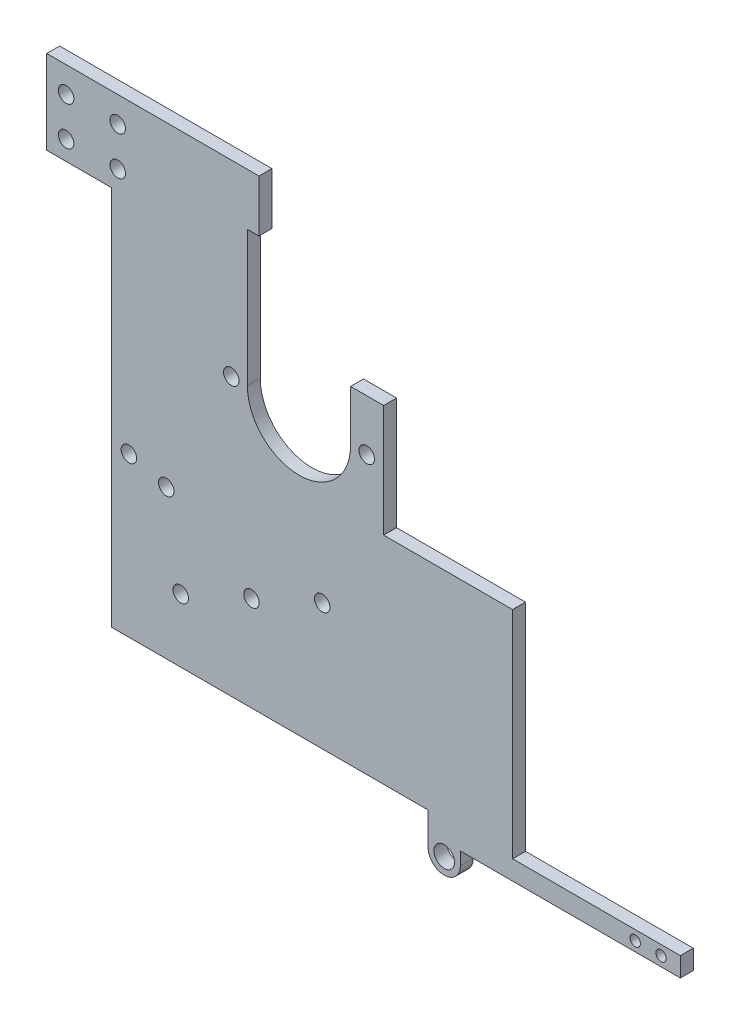
SolidWorks part; units mm, degrees
ref_plane "前视基准面" through (0, 0, 0) normal (0, 0, 1) x (1, 0, 0)
ref_plane "上视基准面" through (0, 0, 0) normal (0, 1, 0) x (1, 0, 0)
ref_plane "右视基准面" through (0, 0, 0) normal (1, 0, 0) x (0, 0, -1)
sketch "草图1" plane through (0, 0, 0) normal (0, 0, 1) x (1, 0, 0)
  line L0 (-200.9973, -87.2636) -> (110, -87.2636)
  line L1 (110, 0) -> (110, 79.9839)
  line L2 (110, 79.9839) -> (85.0706, 79.9839)
  line L3 (85.0706, 79.9839) -> (85.0706, 49.9839)
  line L4 (-200.9973, 332.6816) -> (-250.9973, 332.6816)
  line L5 (25.0706, 49.9839) -> (25.0706, 79.9839)
  line L6 (25.0706, 79.9839) -> (10.0706, 79.9839)
  line L7 (10.0706, 79.9839) -> (10.0706, 166.9839)
  line L8 (110, -87.2636) -> (110, 0)
  line L9 (10.0706, 166.9839) -> (-15.5149, 166.9839)
  line L10 (-15.5149, 166.9839) -> (-15.5149, 127.4167)
  line L11 (-95.5149, 127.4167) -> (-95.5149, 232.4167)
  line L12 (-95.5149, 232.4167) -> (-86.5149, 232.4167)
  line L13 (-250.9973, 332.6816) -> (-250.9973, 212.6816)
  line L14 (-250.9973, 212.6816) -> (-250.9973, 207.6816)
  line L15 (-86.5149, 232.4167) -> (-86.5149, 332.4167)
  line L16 (-86.5149, 332.4167) -> (-110.9973, 332.4167)
  line L17 (-110.9973, 332.4167) -> (-110.9973, 302.6816)
  line L18 (-170.9973, 302.6816) -> (-170.9973, 332.6816)
  line L19 (-170.9973, 332.6816) -> (-200.9973, 332.6816)
  line L20 (-200.9973, 182.6816) -> (-200.9973, -44.6495)
  line L21 (-200.9973, 182.6816) -> (-200.9973, 207.6816)
  line L22 (-200.9973, -44.6495) -> (-200.9973, -87.2636)
  line L23 (-250.9973, 207.6816) -> (-200.9973, 207.6816)
  arc A0 (25.0706, 49.9839) -> (85.0706, 49.9839) centre (55.0706, 49.9839) ccw
  arc A1 (-95.5149, 127.4167) -> (-15.5149, 127.4167) centre (-55.5149, 127.4167) ccw
  arc A2 (-170.9973, 302.6816) -> (-110.9973, 302.6816) centre (-140.9973, 302.6816) ccw
  circle A3 centre (96.0706, 49.9839) radius 5
  circle A4 centre (14.0706, 49.9839) radius 5
  circle A5 centre (-3.0149, 127.4167) radius 6
  circle A6 centre (-108.0149, 127.4167) radius 6
  circle A7 centre (-99.9973, 302.6816) radius 5
  circle A8 centre (-181.9973, 302.6766) radius 5
  circle A9 centre (-37.5239, 10.6592) radius 6
  circle A10 centre (-92.3366, -13.745) radius 6
  circle A11 centre (-147.1493, -38.1492) radius 6
  circle A12 centre (-235.9973, 222.6816) radius 6
  circle A13 centre (-195.9995, 222.6816) radius 6
  circle A14 centre (-235.9973, 252.6816) radius 6
  circle A15 centre (-195.9973, 252.6816) radius 6
  dimension "D1" = 41
  dimension "D2" = 41
  dimension "D3" = 15
  dimension "D4" = 52.5
  dimension "D5" = 52.5
  dimension "D6" = 41
  dimension "D7" = 41
  dimension "D9" = 15
  dimension "D10" = 60
  dimension "D11" = 60
  dimension "D8" = 30
  dimension "D12" = 45
  dimension "D14" = 40
  dimension "D17" = 15
extrude "凸台-拉伸1" add sketch "草图1" along normal blind 10
sketch "草图2" plane through (0, 0, 10) normal (0, 0, 1) x (1, 0, 0)
  circle A0 centre (-158.3587, 28.0551) radius 6
  circle A1 centre (-187.3364, 35.8196) radius 6
extrude "切除-拉伸1" cut sketch "草图2" against normal blind 10
sketch "草图3" plane through (0, 0, 10) normal (0, 0, 1) x (1, 0, 0)
  line L0 (110, -87.2636) -> (62, -87.2636)
  line L1 (-200.9973, -87.2636) -> (110, -87.2636) construction
  line L2 (110, -87.2636) -> (240, -87.2636)
  line L3 (44.5, -112.2636) -> (44.5, -87.2636)
  line L4 (44.5, -87.2636) -> (62, -87.2636)
  line L5 (69.5, -112.2636) -> (69.5, -102.2636)
  line L6 (69.5, -102.2636) -> (240, -102.2636)
  line L7 (240, -102.2636) -> (240, -87.2636)
  circle A0 centre (57, -112.2636) radius 8
  arc A1 (44.5, -112.2636) -> (69.5, -112.2636) centre (57, -112.2636) ccw
  circle A2 centre (225, -94.7636) radius 4
  circle A3 centre (205, -94.7636) radius 4
  dimension "D1" = 15
  dimension "D2" = 20
extrude "凸台-拉伸2" add sketch "草图3" against normal blind 10
sketch "草图4" plane through (0, 0, 0) normal (0, 0, -1) x (-1, 0, 0)
  line L0 (140.9973, 272.6816) -> (86.5149, 272.6816)
  line L1 (86.5149, 232.4167) -> (86.5149, 332.4167) construction
  line L2 (140.9973, 272.6816) -> (250.9973, 272.6816)
  line L3 (250.9973, 332.6816) -> (250.9973, 207.6816) construction
  arc A0 (110.9973, 302.6816) -> (170.9973, 302.6816) centre (140.9973, 302.6816) ccw construction
extrude "切除-拉伸3" cut sketch "草图4" against normal blind 10 and the other way through all
sketch "草图5" plane through (0, 0, 0) normal (0, 0, -1) x (-1, 0, 0)
  circle A0 centre (-96.0706, 49.9839) radius 5
extrude "凸台-拉伸3" add sketch "草图5" against normal blind 10
sketch "草图6" plane through (0, 0, 0) normal (0, 0, -1) x (-1, 0, 0)
  circle A0 centre (-14.0706, 49.9839) radius 5
extrude "凸台-拉伸4" add sketch "草图6" against normal blind 10
sketch "草图7" plane through (0, 0, 0) normal (0, 0, -1) x (-1, 0, 0)
  line L0 (-85.0706, 79.9839) -> (-85.0706, 49.9839)
  line L1 (-25.0706, 79.9839) -> (-85.0706, 79.9839)
  line L2 (-25.0706, 79.9839) -> (-25.0706, 49.9839)
  arc A2 (-85.0706, 49.9839) -> (-25.0706, 49.9839) centre (-55.0706, 49.9839) ccw
extrude "凸台-拉伸5" add sketch "草图7" against normal blind 10
